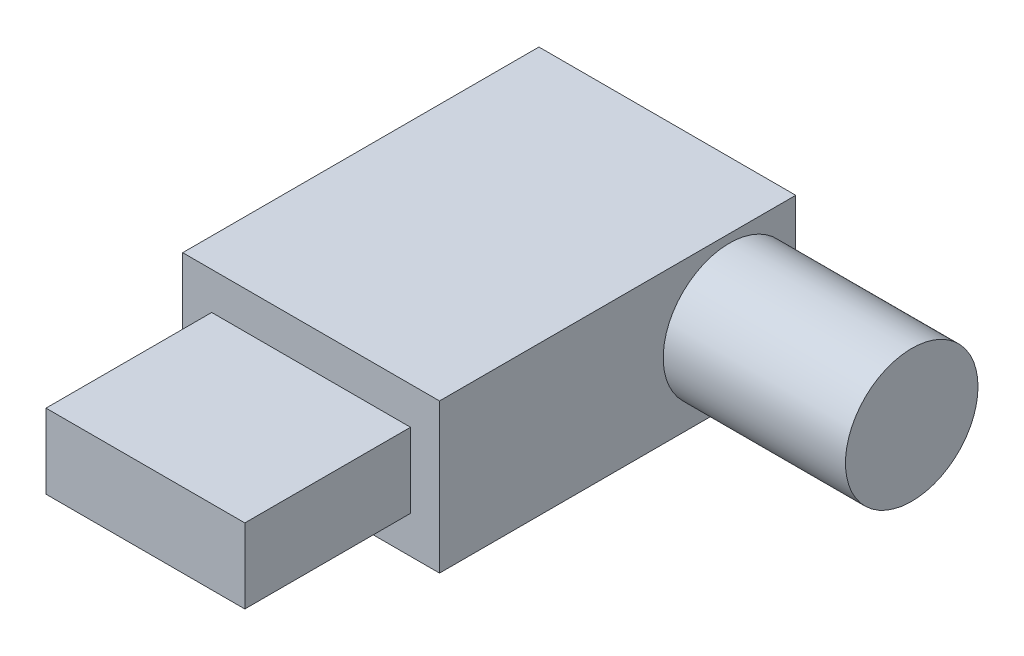
SolidWorks part; units mm, degrees
ref_plane "Front Plane" through (0, 0, 0) normal (0, 0, 1) x (1, 0, 0)
ref_plane "Top Plane" through (0, 0, 0) normal (0, 1, 0) x (1, 0, 0)
ref_plane "Right Plane" through (0, 0, 0) normal (1, 0, 0) x (0, 0, -1)
sketch "Sketch1" plane through (0, 0, 0) normal (0, 0, 1) x (1, 0, 0)
  line L1 (-7.75, -4.5) -> (7.75, -4.5)
  line L2 (-7.75, -4.5) -> (-7.75, 4.5)
  line L3 (-7.75, 4.5) -> (7.75, 4.5)
  line L4 (7.75, -4.5) -> (7.75, 4.5)
  line L5 (-7.75, -4.5) -> (7.75, 4.5) construction
  line L6 (-7.75, 4.5) -> (7.75, -4.5) construction
  point P0 (0, 0)
  dimension "D1" = 15.5
  dimension "D2" = 9
extrude "Boss-Extrude1" add sketch "Sketch1" against normal blind 21.5
sketch "Sketch2" plane through (7.75, 0, 0) normal (1, 0, 0) x (0, 0, -1)
  line L0 (0, 0) -> (21.5, 0) construction
  line L1 (21.5, -4.5) -> (21.5, 4.5) construction
  circle A0 centre (17.5, 0) radius 4
  dimension "D1" = 8
  dimension "D2" = 4
extrude "Boss-Extrude2" add sketch "Sketch2" along normal blind 11
sketch "Sketch3" plane through (0, 0, 0) normal (0, 0, 1) x (1, 0, 0)
  line L1 (-6, -2.25) -> (6, -2.25)
  line L2 (-6, -2.25) -> (-6, 2.25)
  line L3 (-6, 2.25) -> (6, 2.25)
  line L4 (6, -2.25) -> (6, 2.25)
  line L5 (-6, -2.25) -> (6, 2.25) construction
  line L6 (-6, 2.25) -> (6, -2.25) construction
  point P0 (0, 0)
  dimension "D1" = 12
  dimension "D2" = 4.5
extrude "Boss-Extrude3" add sketch "Sketch3" along normal blind 10
